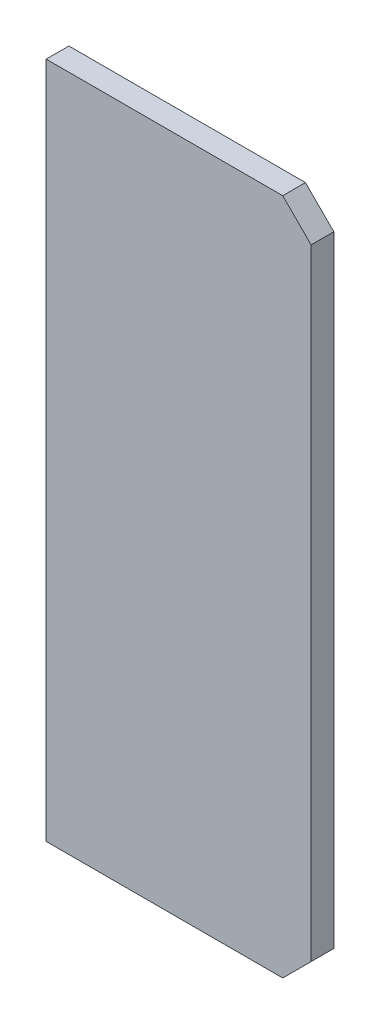
SolidWorks part; units mm, degrees
material "Q235"
ref_plane "Front Plane" through (0, 0, 0) normal (0, 0, 1) x (1, 0, 0)
ref_plane "Top Plane" through (0, 0, 0) normal (0, 1, 0) x (1, 0, 0)
ref_plane "Right Plane" through (0, 0, 0) normal (1, 0, 0) x (0, 0, -1)
sketch "Sketch1" plane through (0, 0, 0) normal (0, 0, 1) x (1, 0, 0)
  line L1 (0, 0) -> (140, 0)
  line L2 (0, 0) -> (0, 358)
  line L3 (0, 358) -> (140, 358)
  line L4 (140, 0) -> (140, 358)
  dimension "D1" = 140
  dimension "D2" = 358
extrude "Boss-Extrude1" add sketch "Sketch1" along normal blind 12
chamfer "Chamfer2" distance 15 angle 45 2 edges at (140, 0, 6) (140, 358, 6)
